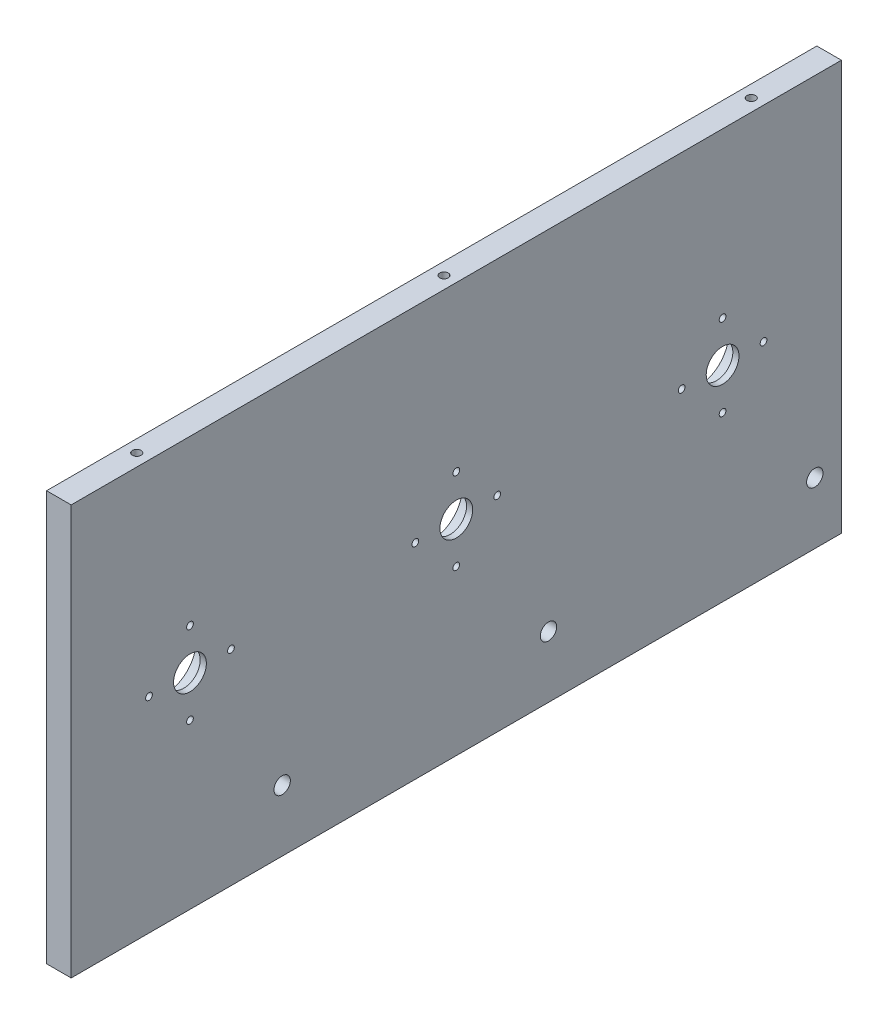
from build123d import *

# Parameters (mm, degrees)
SKETCH1_W                  = 376
SKETCH1_H                  = 200
BOSS_EXTRUDE1_DEPTH        = 6
M5_TAPPED_HOLE1_AT_2_COUNT = 2
M5_TAPPED_HOLE1_AT_2_PITCH = 300
M5_TAPPED_HOLE1_AT_3_COUNT = 2
M5_TAPPED_HOLE1_AT_3_PITCH = 150
SKETCH4_R                  = 15
CUT_EXTRUDE1_DEPTH         = 9
SKETCH6_R                  = 8
CUT_EXTRUDE2_DEPTH         = 214.279159788
M4_TAPPED_HOLE1_D          = 3.3
SKETCH9_R                  = 4
CUT_EXTRUDE3_DEPTH         = 214.279159788


with BuildPart() as part:
    # Sketch1 → Boss-Extrude1 (new, symmetric)
    with BuildSketch(Plane(origin=(0, 0, 0), x_dir=(0, 0, -1), z_dir=(1, 0, 0))):
        Rectangle(SKETCH1_W, SKETCH1_H)
    extrude(amount=BOSS_EXTRUDE1_DEPTH, both=True)

    # Sketch3 → M5 Tapped Hole1 (revolve, cut)
    with BuildSketch(Plane(origin=(0, 100, -150), x_dir=(0, 0, 1), z_dir=(1, 0, 0))):
        Polygon((0, 0), (0, 25.7618073), (2.1, 24.5), (2.1, 0), align=None)
    m5_tapped_hole1 = revolve(axis=Axis((0, 106.35, -150), (0, -1, 0)), mode=Mode.SUBTRACT)

    # M5 Tapped Hole1 at 2: M5 Tapped Hole1 ×2
    with Locations(*[(0, 0, i * M5_TAPPED_HOLE1_AT_2_PITCH) for i in range(1, M5_TAPPED_HOLE1_AT_2_COUNT)]):
        add(m5_tapped_hole1, mode=Mode.SUBTRACT)

    # M5 Tapped Hole1 at 3: M5 Tapped Hole1 ×2
    with Locations(*[(0, 0, i * M5_TAPPED_HOLE1_AT_3_PITCH) for i in range(1, M5_TAPPED_HOLE1_AT_3_COUNT)]):
        add(m5_tapped_hole1, mode=Mode.SUBTRACT)

    # Mirror1: M5 Tapped Hole1 across plane
    add(m5_tapped_hole1.mirror(Plane.ZX), mode=Mode.SUBTRACT)

    # Mirror1 copy 1 sketch → Mirror1 copy 1 (revolve, cut)
    with BuildSketch(Plane(origin=(0, -100, 150), x_dir=(0, 0, 1), z_dir=(1, 0, 0))):
        Polygon((0, 0), (0, -25.7618073), (2.1, -24.5), (2.1, 0), align=None)
    revolve(axis=Axis((0, -106.35, 150), (0, -1, 0)), mode=Mode.SUBTRACT)

    # Mirror1 copy 2 sketch → Mirror1 copy 2 (revolve, cut)
    with BuildSketch(Plane(origin=(0, -100, 0), x_dir=(0, 0, 1), z_dir=(1, 0, 0))):
        Polygon((0, 0), (0, -25.7618073), (2.1, -24.5), (2.1, 0), align=None)
    revolve(axis=Axis((0, -106.35, 0), (0, -1, 0)), mode=Mode.SUBTRACT)

    # Sketch4 → Cut-Extrude1 (cut)
    with BuildSketch(Plane.ZY.offset(6)):
        with Locations((-130, 0)):
            Circle(SKETCH4_R)
        Circle(SKETCH4_R)
        with Locations((130, 0)):
            Circle(SKETCH4_R)
    extrude(amount=-CUT_EXTRUDE1_DEPTH, mode=Mode.SUBTRACT)

    # Sketch6 → Cut-Extrude2 (cut, through all)
    with BuildSketch(Plane.ZY.offset(6)):
        with Locations((-130, 0)):
            Circle(SKETCH6_R)
        Circle(SKETCH6_R)
        with Locations((130, 0)):
            Circle(SKETCH6_R)
    extrude(amount=-CUT_EXTRUDE2_DEPTH, mode=Mode.SUBTRACT)

    # M4 Tapped Hole1 (through all)
    with Locations(Plane.ZY.offset(6)):
        with Locations((130, -20), (-150, 0), (-130, 20), (-110, 0), (-130, -20), (-20, 0), (0, 20), (20, 0), (0, -20), (110, 0), (130, 20), (150, 0)):
            Hole(M4_TAPPED_HOLE1_D / 2)

    # Sketch9 → Cut-Extrude3 (cut, through all)
    with BuildSketch(Plane.ZY.offset(6)):
        with Locations((-175, -70)):
            Circle(SKETCH9_R)
        with Locations((-45, -70)):
            Circle(SKETCH9_R)
        with Locations((85, -70)):
            Circle(SKETCH9_R)
    extrude(amount=-CUT_EXTRUDE3_DEPTH, mode=Mode.SUBTRACT)


solid = part.part
